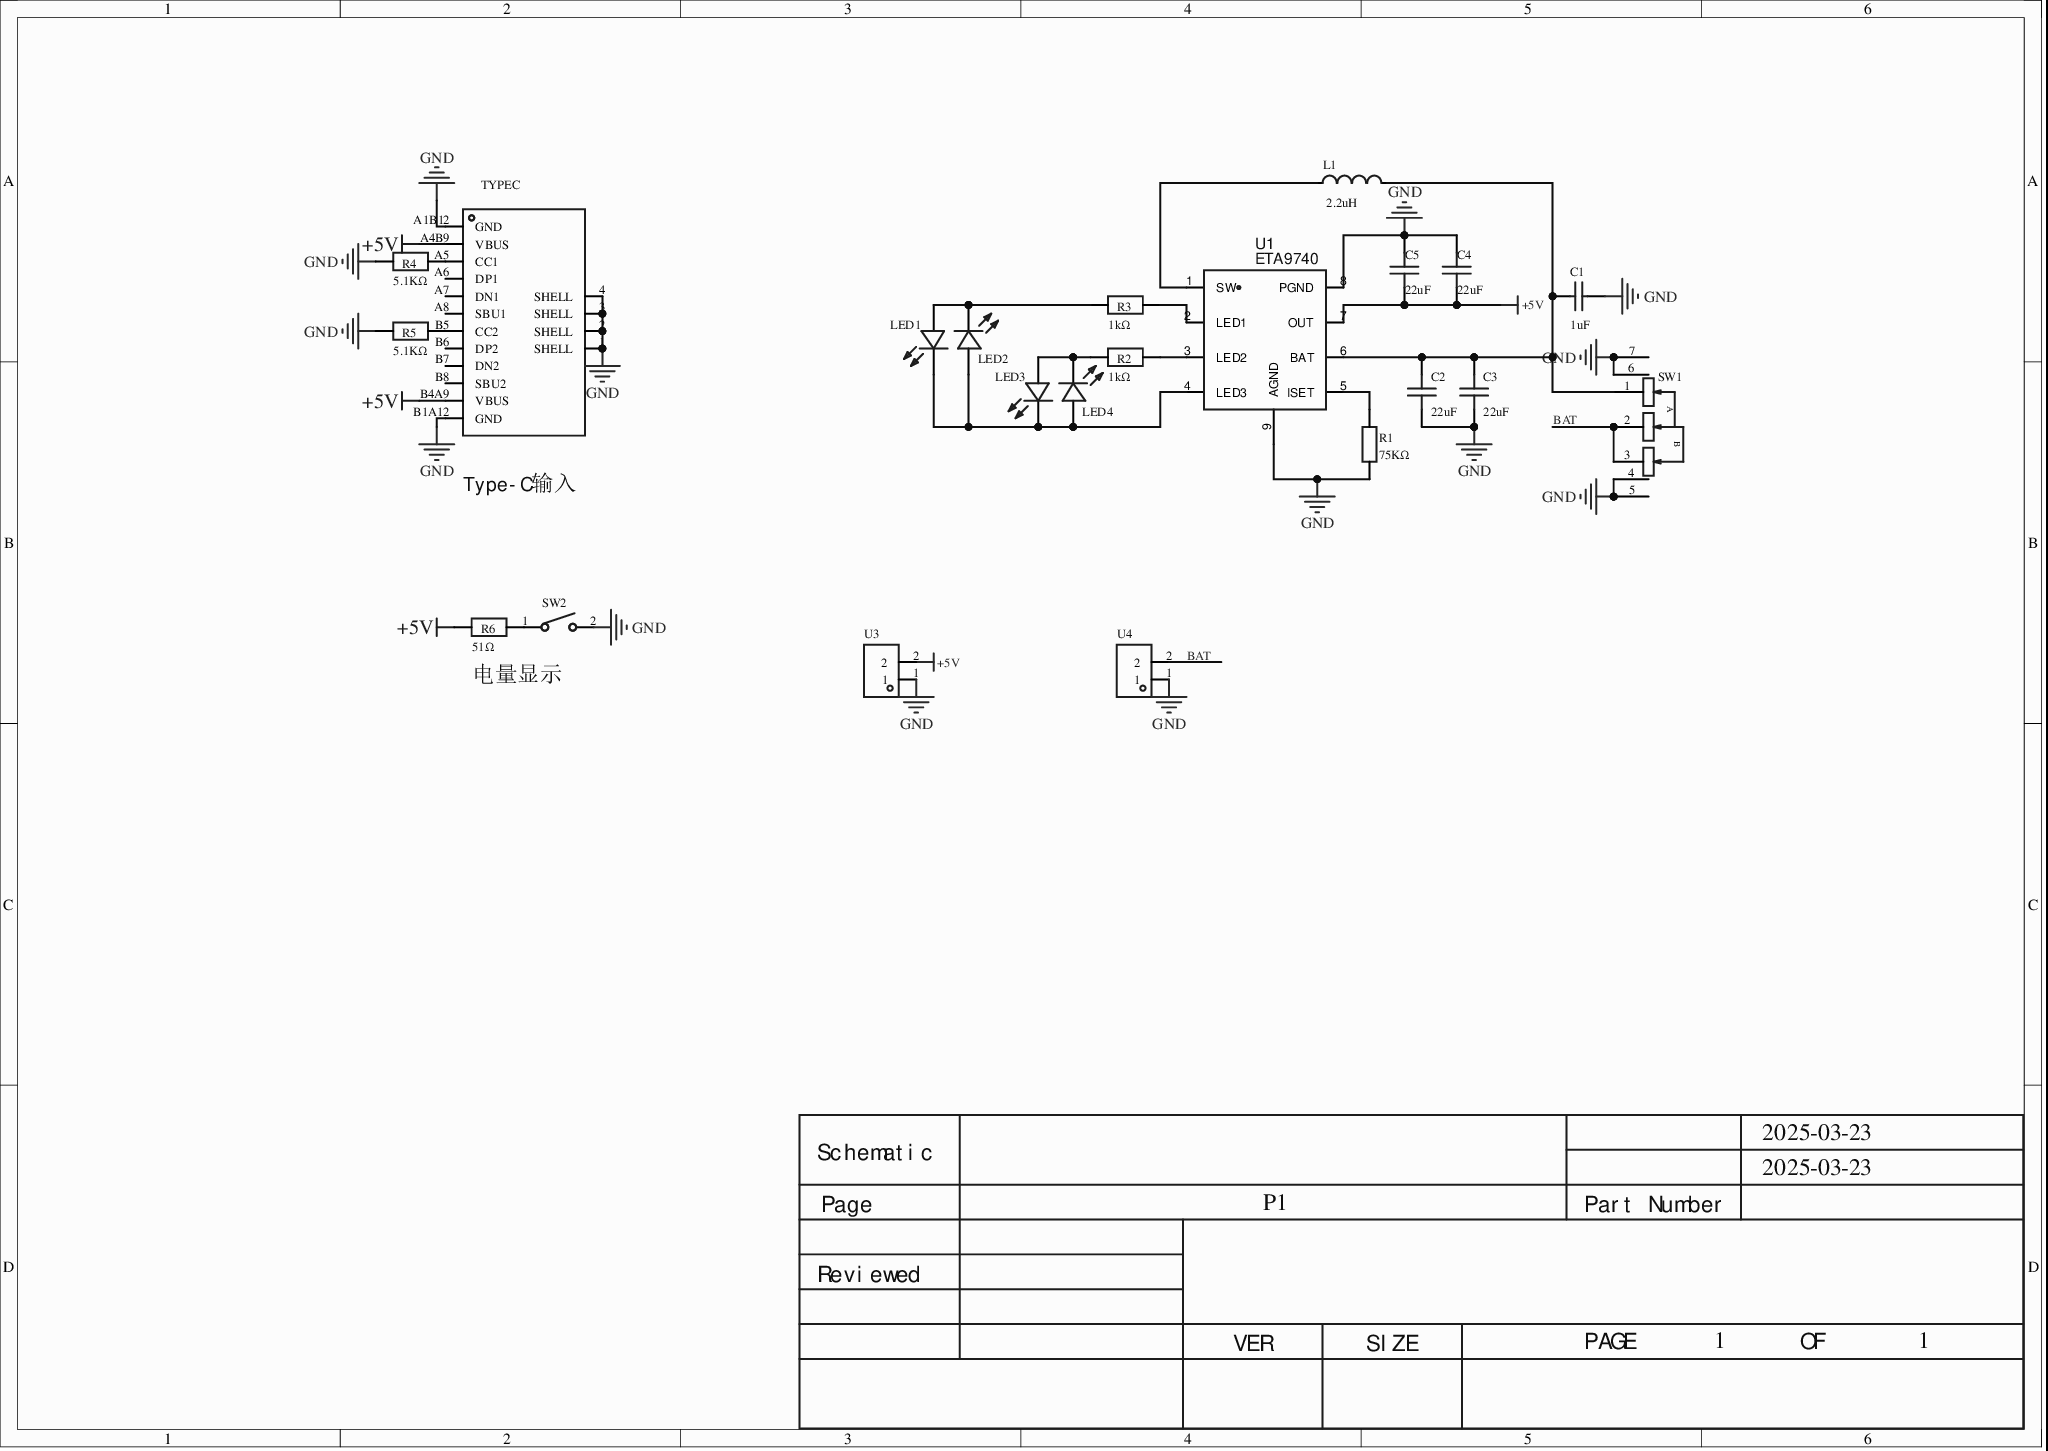
[diagram p0: MISC51179-3.schdoc]
# Altium project MISC51179.PrjPcb
1 sheet, 22 parts. Net scope: global (net labels, ports and power ports of the same name join across sheets).
Board file: MISC51179.pcbdoc

## Sheet MISC51179-3.schdoc
size 297 x 210 mm; @Project Name: MISC51179; @Page Count: 1; @Update Date: 2025-03-23; @Create Date: 2025-03-23; @Schematic Name: MISC51179; @Page No: 1

### Parts
C1  value 1uF  [C0805]  (hidden comment: CL21B105KBFNNNE)
C2  value 22uF  [C0805]  (hidden comment: CL21A226MAQNNNE_C45783)
C3  value 22uF  [C0805]  (hidden comment: CL21A226MAQNNNE_C45783)
C4  value 22uF  [C0805]  (hidden comment: CL21A226MAQNNNE_C45783)
C5  value 22uF  [C0805]  (hidden comment: CL21A226MAQNNNE_C45783)
L1  value 2.2uH  [IND-SMD_L5.4-W5.2]  (hidden comment: YTA0520-2R2M)
LED1  led0805  [LED0805-RD]  (value not drawn)
LED2  led0805  [LED0805-RD]  (value not drawn)
LED3  led0805  [LED0805-RD]  (value not drawn)
LED4  led0805  [LED0805-RD]  (value not drawn)
R1  value 75KΩ  [R0805]  (hidden comment: AC0805JR-07100KL)
R2  value 1kΩ  [R0805]  (hidden comment: RT0805CRE071KL)
R3  value 1kΩ  [R0805]  (hidden comment: RT0805CRE071KL)
R4  value 5.1KΩ  [R0805]  (hidden comment: RT0805CRE071KL)
R5  value 5.1KΩ  [R0805]  (hidden comment: RT0805CRE071KL)
R6  value 51Ω  [R0805]  (hidden comment: RT0805CRE071KL)
SW1  MK-12C02-G015  [SW-SMD_G-SWITCH_MK-12C02-G015]  (value not drawn)
SW2  ST-1185U  [SW-SMD_ST-1185U]  (value not drawn)
TYPEC  TYPE-C 16PIN 3MD(385)  [USB-C-SMD_TYPE-C16PIN]  (value not drawn)
U1  ETA9740  [ESOP-8]
U3  2.54-1*2  [HDR-TH_2P-P2.54-V-M]  (value not drawn)
U4  2.54-1*2  [HDR-TH_2P-P2.54-V-M]  (value not drawn)

### Nets
+5V: C4.2 C5.2 R6.1 TYPEC.A4B9(VBUS) TYPEC.B4A9(VBUS) U1.7(OUT) U3.2
GND: C1.2 C2.1 C3.1 C4.1 C5.1 R1.1 R4.1 R5.1 SW1.4 SW1.5 SW1.6 SW1.7 SW2.2 TYPEC.1(SHELL) TYPEC.2(SHELL) TYPEC.3(SHELL) TYPEC.4(SHELL) TYPEC.A1B12(GND) TYPEC.B1A12(GND) U1.8(PGND) U1.9(AGND) U3.1 U4.1
BAT: SW1.2 SW1.3 U4.2
NetC1_1: C1.1 C2.2 C3.2 L1.2 SW1.1 U1.6(BAT)
NetL1_1: L1.1 U1.1(SW)
NetLED1_1: LED1.1(-) LED2.2(+) LED3.1(-) LED4.2(+) U1.4(LED3)
NetLED1_2: LED1.2(+) LED2.1(-) R3.1
NetLED3_2: LED3.2(+) LED4.1(-) R2.1
NetR1_2: R1.2 U1.5(ISET)
NetR2_2: R2.2 U1.3(LED2)
NetR3_2: R3.2 U1.2(LED1)
NetR4_2: R4.2 TYPEC.A5(CC1)
NetR5_2: R5.2 TYPEC.B5(CC2)
NetR6_2: R6.2 SW2.1

Not connected (* = marked no-connect by the designer): TYPEC A6(DP1)* A7(DN1)* A8(SBU1)* B6(DP2)* B7(DN2)* B8(SBU2)*

### Notes on the sheet
- (near TYPEC) Type-C输入
- 电量显示
- 2025-03-23
- Schematic
- Page
- P1
- Part Number
- Reviewed
- VER
- SIZE
- PAGE
- 1
- OF

### Library data of the parts
C1 = CL21B105KBFNNNE: 容值:1uF;精度:±10%;额定电压:50V;材质(温度系数):X7R;; Manufacturer: SAMSUNG(三星); AddInBom: yes; ModelId: 1ba041120af144c991958decab20d241; ModelName: C0805_L2.0-W1.3-H1.3; ModelTransform: 78.74,51.181,0,0,0,0,0,0.0005,0; Tolerance: ±10%; Voltage Rated: 50V; Temperature Coefficient: X7R; Device: CL21B105KBFNNNE; Symbol: CL21B105KBFNNNE; LCSC Part Name: 1uF ±10% 50V; SupplierPart: C28323; ManufacturerPart: CL21B105KBFNNNE; Supplier Footprint: 0805; JLCPCB Part Class: Basic Part; Datasheet: https://atta.szlcsc.com/upload/public/pdf/source/20160103/1457707718219.pdf; Supplier: LCSC; ConvertToPcb: yes; FootprintName: C0805
C2-C5 = CL21A226MAQNNNE_C45783: 容值:22uF;精度:±20%;额定电压:25V;温度系数:X5R;; Manufacturer: SAMSUNG(三星); AddInBom: yes; ModelId: 1ba041120af144c991958decab20d241; ModelName: C0805_L2.0-W1.3-H1.3; ModelTransform: 78.74,51.181,0,0,0,0,0,0.0005,0; Tolerance: ±20%; Voltage Rated: 25V; Temperature Coefficient: X5R; Symbol: CL21A226MAQNNNE; Device: CL21A226MAQNNNE_C45783; LCSC Part Name: 22uF ±20% 25V; SupplierPart: C45783; ManufacturerPart: CL21A226MAQNNNE; Supplier Footprint: 0805; JLCPCB Part Class: Basic Part; Datasheet: https://atta.szlcsc.com/upload/public/pdf/source/20160103/1457707727161.pdf; Supplier: LCSC; ConvertToPcb: yes; FootprintName: C0805
L1 = YTA0520-2R2M: 电感值:2.2uH;精度:±20%;额定电流:5A;直流电阻(DCR):34mΩ;; Manufacturer: Wenshan(文善); AddInBom: yes; ModelId: 8cf4ba96105a43709c0ba3ecbf611559; ModelName: IND-SMD_L5.4-W5.2-H3.0; ModelTransform: 212.598,204.724,0,0,0,0,0,0,0; Tolerance: ±20%; Rated Current: 5A; DC Resistance (DCR): 34mΩ; Device: YTA0520-2R2M; Symbol: YTA0520-2R2M; LCSC Part Name: 2.2uH ±20% 5A 34mΩ; SupplierPart: C428590; ManufacturerPart: YTA0520-2R2M; Supplier Footprint: SMD; JLCPCB Part Class: Extended Part; Datasheet: https://atta.szlcsc.com/upload/public/pdf/source/20190912/C428590_7213E84AF1EC908B0D3C5640122957DB.pdf; Supplier: LCSC; ConvertToPcb: yes; FootprintName: IND-SMD_L5.4-W5.2
LED1-LED4 = led0805: AddInBom: yes; ModelId: 23093642268545519703b953fc993978; ModelTransform: 79.527,49.2125,0,0,0,0,0,0,0; Symbol: LED0805; Device: led0805; LCSC Part Name: led0805; SupplierPart: C9900012722; ManufacturerPart: led0805; Supplier Footprint: led0805; JLCPCB Part Class: Extended Part; Datasheet: https://atta.szlcsc.comnull; Supplier: LCSC; ConvertToPcb: yes; FootprintName: LED0805-RD; ModelName: LED0805-RD
R1 = AC0805JR-07100KL: 电阻类型:厚膜电阻;阻值:100kΩ;精度:±5%;功率:125mW;温度系数:±100ppm/;最大工作电压:150V;工作温度范围:-55~+155;; Manufacturer: YAGEO(国巨); AddInBom: yes; ModelId: 37a81e68749a4138bd2dfa6897b24b85; ModelName: R0805_L2.0-W1.3-H0.6; ModelTransform: 78.74,51.181,0,0,0,0,0,-0.0005,0; Tolerance: ±5%; Power(Watts): 125mW; Overload Voltage (Max): 150V; Symbol: AC0805JR-07100KL; Temperature Coefficient: ±100ppm/; Operating Temperature Range: -55~+155; Device: AC0805JR-07100KL; LCSC Part Name: 100kΩ ±5%; SupplierPart: C138261; ManufacturerPart: AC0805JR-07100KL; Supplier Footprint: 0805; JLCPCB Part Class: Extended Part; Datasheet: https://atta.szlcsc.com/upload/public/pdf/source/20171107/C138261_15100517928971097152.pdf; Supplier: LCSC; ConvertToPcb: yes; FootprintName: R0805; Type: 厚膜电阻
R2-R6 = RT0805CRE071KL: 电阻类型:薄膜电阻;阻值:1kΩ;精度:±0.25%;功率:125mW;温度系数:±50ppm/;最大工作电压:150V;工作温度范围:-55~+155;; Manufacturer: YAGEO(国巨); Temperature Coefficient: ±50ppm/; AddInBom: yes; ModelId: 37a81e68749a4138bd2dfa6897b24b85; ModelName: R0805_L2.0-W1.3-H0.6; ModelTransform: 78.74,51.181,0,0,0,0,0,-0.0005,0; Tolerance: ±0.25%; Power(Watts): 125mW; Overload Voltage (Max): 150V; Operating Temperature Range: -55~+155; Device: RT0805CRE071KL; Symbol: RT0805CRE071KL; LCSC Part Name: 1kΩ ±0.25% 125mW; SupplierPart: C706297; ManufacturerPart: RT0805CRE071KL; Supplier Footprint: 0805; JLCPCB Part Class: Extended Part; Datasheet: https://atta.szlcsc.com/upload/public/pdf/source/20200720/C706297_0975DDBB81B75BFD1E18A877B21309C0.pdf; Supplier: LCSC; ConvertToPcb: yes; FootprintName: R0805; Type: 薄膜电阻
SW1 = MK-12C02-G015: Manufacturer: G-Switch(品赞); AddInBom: yes; ModelId: 1349463526a14cfbb2c214633ebf018b; ModelName: SW-SMD_MK-12C02-G020; ModelTransform: 307.086,200.787,0,0,0,0,0,-25.894,-19.685; Symbol: MK-12C02-G015; Supplier Footprint: SMD,6.62.71.4mm; Device: MK-12C02-G015; LCSC Part Name: 七脚贴片微型拨动开关 G1.5; SupplierPart: C2911519; ManufacturerPart: MK-12C02-G015; JLCPCB Part Class: Extended Part; Datasheet: https://atta.szlcsc.com/upload/public/pdf/source/20200902/C778186_2AF08473ED98414D93A175E8814EEFA6.pdf; Supplier: LCSC; ConvertToPcb: yes; FootprintName: SW-SMD_G-SWITCH_MK-12C02-G015
SW2 = ST-1185U: 触点电流:50mA;额定电压(DC):12V;绝缘电阻:100MΩ;电路结构:单刀单掷;安装方式:立贴;按钮形状:圆形按钮;按钮/盖帽颜色:黑色;机械寿命:100000;工作温度:-20~+70;引脚样式:J型引脚;开关长度:4mm;开关宽度:3mm;开关高度:2mm;带支架:否;; Manufacturer: RISHENG(日昇); AddInBom: yes; ModelId: d33132a8fd3d4f24882cba241305d46b; ModelTransform: 173.2,118.1,0,0,0,0,0.3,0,0; Contact Current: 50mA; Voltage Rating (DC): 12V; Insulation Resistance: 100MΩ; Circuit: 单刀单掷; Actuator Style: 圆形按钮; Actuator/Cap Color: 黑色; Mechanical Life: 100000; Pin Style: J型引脚; Switch Length: 4mm; Switch Width: 3mm; Switch Height: 2mm; Strike Gundam: 否; Operating Temperature: -20~+70; Device: ST-1185U; Symbol: ST-1185U; LCSC Part Name: 轻触开关正按小龟; SupplierPart: C589194; ManufacturerPart: ST-1185U; Supplier Footprint: SMD; JLCPCB Part Class: Extended Part; Datasheet: https://atta.szlcsc.com/upload/public/pdf/source/20200922/C589194_60746A96EC0C4390ABA76F9B9AA3C588.pdf; Supplier: LCSC; ConvertToPcb: yes; FootprintName: SW-SMD_ST-1185U; ModelName: SW-SMD_ST-1185U; Mounting Style: 立贴
TYPEC = TYPE-C 16PIN 3MD(385): 连接器类型:Type-C;标准:-;公母:母座;触点数量:16;端口数量:1;安装方式:卧贴;额定电流 - 电源:3A;工作温度范围:-40~+85;; Manufacturer: SHOU HAN(首韩); AddInBom: yes; ModelId: d6783d3a2268456b863f42d3286191d0; ModelTransform: 352,311,0,180,0,0,0,-41.8,-39.4; Gender: 母座; Number of Contacts: 16; Number of Ports: 1; Current Rating - Power (Max): 3A; Operating Temperature Range: -40~+85; Device: TYPE-C 16PIN 3MD(385); Symbol: TYPE-C 16PIN 3MD(385); LCSC Part Name: Type-C 母座 卧贴; SupplierPart: C2858270; ManufacturerPart: TYPE-C 16PIN 3MD(385); Supplier Footprint: SMD; JLCPCB Part Class: Extended Part; Datasheet: https://atta.szlcsc.com/upload/public/pdf/source/20210728/C2858270_8CC81AF68E5F7ED0622FE1183F819D00.pdf; Supplier: LCSC; ConvertToPcb: yes; FootprintName: USB-C-SMD_TYPE-C16PIN; ModelName: USB-C-SMD_TYPE-C16PIN; Connector Type: Type-C; Standard: -; Mounting Style: 卧贴
U1 = ETA9740: Manufacturer: 钰泰半导体; Convert to PCB: yes; Origin Footprint: ESOP-8; Device: ETA9740; Symbol: ETA9740; Add into BOM: yes; FootprintName: ESOP-8
U3 U4 = 2.54-1*2: 排针 2.54mm 1x2P 镀金3u; Manufacturer: ZHOURI(洲日); AddInBom: yes; ModelId: e35305ec3aa84b66b849f914b715e73f; ModelName: HDR2.54-M-LI-1X2P; ModelTransform: 200,100,0,0,0,0,0,0,-118.11; Symbol: 2.54-1*2; Device: 2.54-1*2; LCSC Part Name: 排针 2.54mm 1x2P 镀金3u"; SupplierPart: C5116481; ManufacturerPart: 2.54-1*2; Supplier Footprint: 直插,P=2.54mm; JLCPCB Part Class: Extended Part; Datasheet: https://atta.szlcsc.com/upload/public/pdf/source/20220729/DF18AADA08AA3A4F1D3B0508BB8F7248.pdf; Supplier: LCSC; ConvertToPcb: yes; FootprintName: HDR-TH_2P-P2.54-V-M